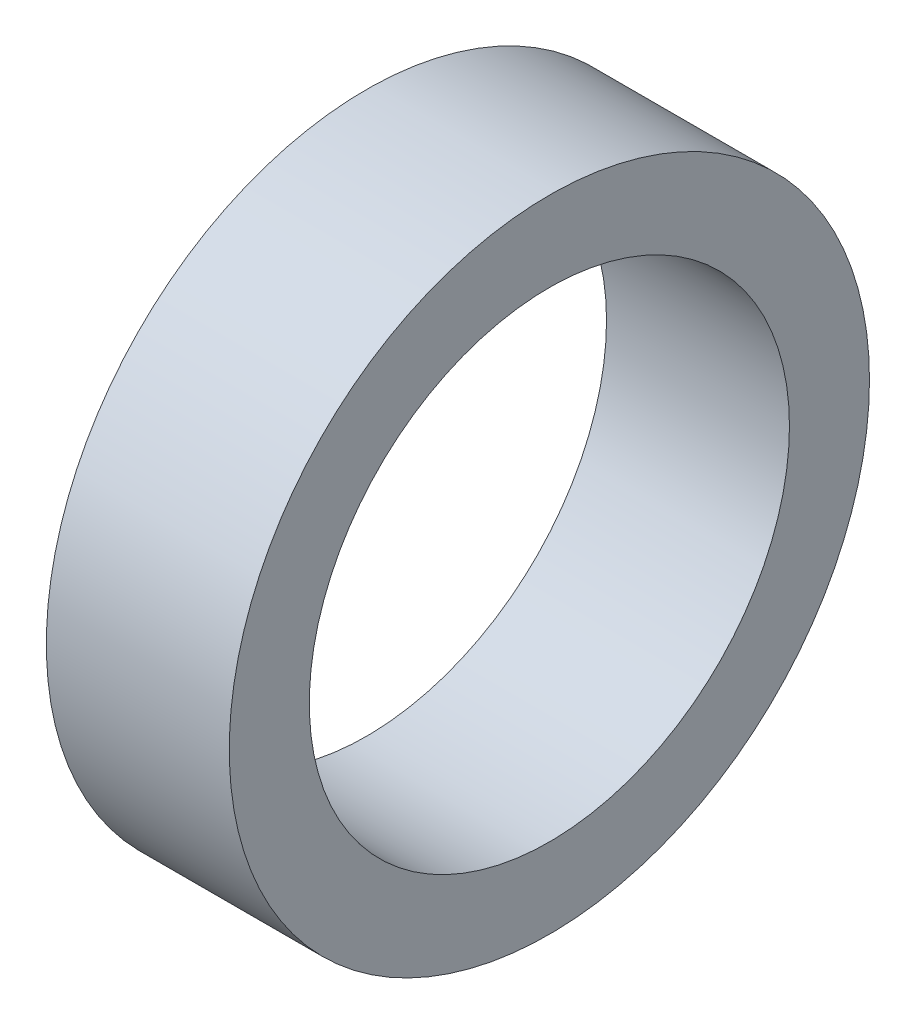
from build123d import *

# Parameters (mm, degrees)
SKETCH_1_R      = 7
SKETCH_1_R_2    = 5.25
EXTRUDE_1_DEPTH = 4


with BuildPart() as part:
    # 草图1 → 凸台-拉伸1 (new body)
    with BuildSketch(Plane(origin=(0, 0, 0), x_dir=(0, 0, -1), z_dir=(1, 0, 0))):
        Circle(SKETCH_1_R)
        Circle(SKETCH_1_R_2, mode=Mode.SUBTRACT)
    extrude(amount=EXTRUDE_1_DEPTH)


solid = part.part
